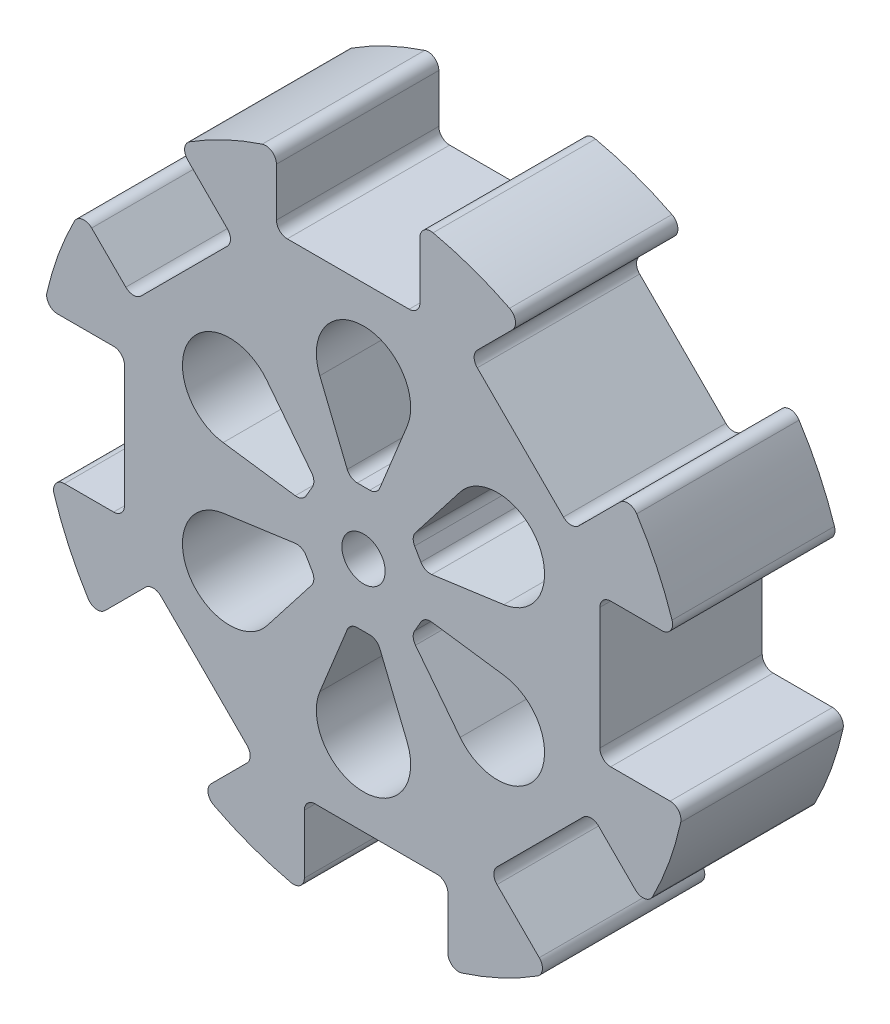
SolidWorks part; units mm, degrees
ref_plane "Front Plane" through (0, 0, 0) normal (0, 0, 1) x (1, 0, 0)
ref_plane "Top Plane" through (0, 0, 0) normal (0, 1, 0) x (1, 0, 0)
ref_plane "Right Plane" through (0, 0, 0) normal (1, 0, 0) x (0, 0, -1)
other "Configuration Table"
sketch "Sketch1" plane through (0, 0, 0) normal (0, 0, 1) x (1, 0, 0)
  line L2 (10.4292, 56.6526) -> (10.4292, 46.1686)
  line L3 (8.4292, 44.1686) -> (-14.0858, 44.1686)
  line L4 (-16.0858, 55.1081) -> (-16.0858, 46.1686)
  line L5 (47.3767, 32.7741) -> (39.7707, 25.168)
  line L7 (27.4956, 50.3908) -> (21.0217, 43.9169)
  line L8 (36.9422, 25.168) -> (21.0217, 41.0885)
  line L9 (56.6526, -10.4292) -> (45.6686, -10.4292)
  line L11 (55.1081, 16.0858) -> (45.6686, 16.0858)
  line L12 (43.6686, -8.4292) -> (43.6686, 14.0858)
  line L13 (32.4689, -47.5716) -> (24.668, -39.7707)
  line L15 (50.2225, -27.8273) -> (43.4169, -21.0217)
  line L16 (24.668, -36.9422) -> (40.5885, -21.0217)
  line L17 (-10.9292, -56.5406) -> (-10.9292, -45.6686)
  line L19 (15.5858, -55.2697) -> (15.5858, -45.6686)
  line L20 (-8.9292, -43.6686) -> (13.5858, -43.6686)
  line L21 (-47.7647, -32.1621) -> (-40.2707, -24.668)
  line L23 (-28.1572, -50.0524) -> (-21.5217, -43.4169)
  line L24 (-37.4422, -24.668) -> (-21.5217, -40.5885)
  line L25 (-56.5406, 10.9292) -> (-46.1686, 10.9292)
  line L27 (-55.2697, -15.5858) -> (-46.1686, -15.5858)
  line L28 (-44.1686, 8.9292) -> (-44.1686, -13.5858)
  line L29 (-32.4689, 47.5716) -> (-25.168, 40.2707)
  line L31 (-50.2225, 27.8273) -> (-43.9169, 21.5217)
  line L32 (-25.168, 37.4422) -> (-41.0885, 21.5217)
  circle A0 centre (0, 0) radius 4
  arc A1 (57.0084, 18.7094) -> (50.4734, 32.4413) centre (0, 0) ccw
  arc A2 (53.4173, -27.3239) -> (58.6061, -12.8578) centre (0, 0) ccw
  arc A3 (18.1922, -57.1756) -> (32.1256, -50.6749) centre (0, 0) ccw
  arc A4 (-27.6652, -53.2413) -> (-13.375, -58.4902) centre (0, 0) ccw
  arc A5 (-53.4173, 27.3239) -> (-58.4902, 13.375) centre (0, 0) ccw
  arc A6 (-57.1756, -18.1922) -> (-50.8748, -31.8082) centre (0, 0) ccw
  arc A7 (-18.7094, 57.0084) -> (-32.1256, 50.6749) centre (0, 0) ccw
  arc A8 (26.9808, 53.5914) -> (12.8578, 58.6061) centre (0, 0) ccw
  arc A9 (-47.7647, -32.1621) -> (-50.8748, -31.8082) centre (-49.1789, -30.7479) cw
  arc A10 (58.6061, -12.8578) -> (56.6526, -10.4292) centre (56.6526, -12.4292) ccw
  arc A11 (55.1081, 16.0858) -> (57.0084, 18.7094) centre (55.1081, 18.0858) ccw
  arc A12 (-25.168, 40.2707) -> (-25.168, 37.4422) centre (-26.5822, 38.8564) cw
  arc A13 (-43.9169, 21.5217) -> (-41.0885, 21.5217) centre (-42.5027, 22.936) ccw
  arc A14 (-46.1686, 10.9292) -> (-44.1686, 8.9292) centre (-46.1686, 8.9292) cw
  arc A15 (-46.1686, -15.5858) -> (-44.1686, -13.5858) centre (-46.1686, -13.5858) ccw
  arc A16 (-40.2707, -24.668) -> (-37.4422, -24.668) centre (-38.8564, -26.0822) cw
  arc A17 (-21.5217, -43.4169) -> (-21.5217, -40.5885) centre (-22.936, -42.0027) ccw
  arc A18 (-32.4689, 47.5716) -> (-32.1256, 50.6749) centre (-31.0547, 48.9858) cw
  arc A19 (-10.9292, -45.6686) -> (-8.9292, -43.6686) centre (-8.9292, -45.6686) cw
  arc A20 (15.5858, -45.6686) -> (13.5858, -43.6686) centre (13.5858, -45.6686) ccw
  arc A21 (-50.2225, 27.8273) -> (-53.4173, 27.3239) centre (-51.6367, 26.4131) ccw
  arc A22 (-56.5406, 10.9292) -> (-58.4902, 13.375) centre (-56.5406, 12.9292) cw
  arc A23 (24.668, -39.7707) -> (24.668, -36.9422) centre (26.0822, -38.3564) cw
  arc A24 (43.4169, -21.0217) -> (40.5885, -21.0217) centre (42.0027, -22.436) ccw
  arc A25 (-55.2697, -15.5858) -> (-57.1756, -18.1922) centre (-55.2697, -17.5858) ccw
  arc A26 (-28.1572, -50.0524) -> (-27.6652, -53.2413) centre (-26.743, -51.4666) ccw
  arc A27 (45.6686, -10.4292) -> (43.6686, -8.4292) centre (45.6686, -8.4292) cw
  arc A28 (45.6686, 16.0858) -> (43.6686, 14.0858) centre (45.6686, 14.0858) ccw
  arc A29 (-10.9292, -56.5406) -> (-13.375, -58.4902) centre (-12.9292, -56.5406) cw
  arc A30 (15.5858, -55.2697) -> (18.1922, -57.1756) centre (17.5858, -55.2697) ccw
  arc A31 (39.7707, 25.168) -> (36.9422, 25.168) centre (38.3564, 26.5822) cw
  arc A32 (21.0217, 43.9169) -> (21.0217, 41.0885) centre (22.436, 42.5027) ccw
  arc A33 (47.3767, 32.7741) -> (50.4734, 32.4413) centre (48.791, 31.3599) cw
  arc A34 (-16.0858, 55.1081) -> (-18.7094, 57.0084) centre (-18.0858, 55.1081) ccw
  arc A35 (32.4689, -47.5716) -> (32.1256, -50.6749) centre (31.0547, -48.9858) cw
  arc A36 (27.4956, 50.3908) -> (26.9808, 53.5914) centre (26.0814, 51.805) ccw
  arc A37 (10.4292, 56.6526) -> (12.8578, 58.6061) centre (12.4292, 56.6526) cw
  arc A38 (10.4292, 46.1686) -> (8.4292, 44.1686) centre (8.4292, 46.1686) cw
  arc A39 (-14.0858, 44.1686) -> (-16.0858, 46.1686) centre (-14.0858, 46.1686) cw
  arc A40 (50.2225, -27.8273) -> (53.4173, -27.3239) centre (51.6367, -26.4131) ccw
  point P40 (-0.25, 0.25)
  point P62 (-52.1196, 29.7244)
  point P65 (-58.9962, 10.9292)
  point P72 (-57.9403, -15.5858)
  point P75 (-30.042, -51.9372)
  point P84 (15.5858, -57.9403)
  point P93 (-16.0858, 57.8035)
  point P98 (29.4052, 52.3004)
  point P107 (52.1196, -29.7244)
  dimension "D1" = 8
  dimension "D2" = 120
  dimension "D3" = 2
  dimension "D4" = 8
extrude "Boss-Extrude2" add sketch "Sketch1" along normal blind 30
sketch "Sketch2" plane through (0, 0, 30) normal (0, 0, 1) x (1, 0, 0)
  line L0 (0, 0) -> (0, 23.973) construction
  line L1 (-2.5, 11.5752) -> (2.5, 11.5752)
  line L2 (-2.5, 11.5752) -> (-8.0728, 25.2776)
  line L4 (2.5, 11.5752) -> (8.0728, 25.2776)
  arc A0 (-8.0728, 25.2776) -> (8.0728, 25.2776) centre (0, 28.5609) cw
  dimension "D2" = 5
extrude "Cut-Extrude2" cut sketch "Sketch2" against normal through all both and the other way through all
fillet "Fillet1" radius 2 2 edges at (2.5, 11.5752, 15) (-2.5, 11.5752, 15)
pattern_circular "CirPattern1" count 6 over 360 about axis through (0, 0, 0) along (0, 0, 1) of "Cut-Extrude2", "Fillet1"
sketch "Sketch12" plane through (0, 0, 0) normal (0, 0, -1) x (-1, 0, 0)
  circle A0 centre (32.1103, -0.5561) radius 0.6834
extrude "Cut-Extrude4" cut sketch "Sketch12" against normal blind 1
